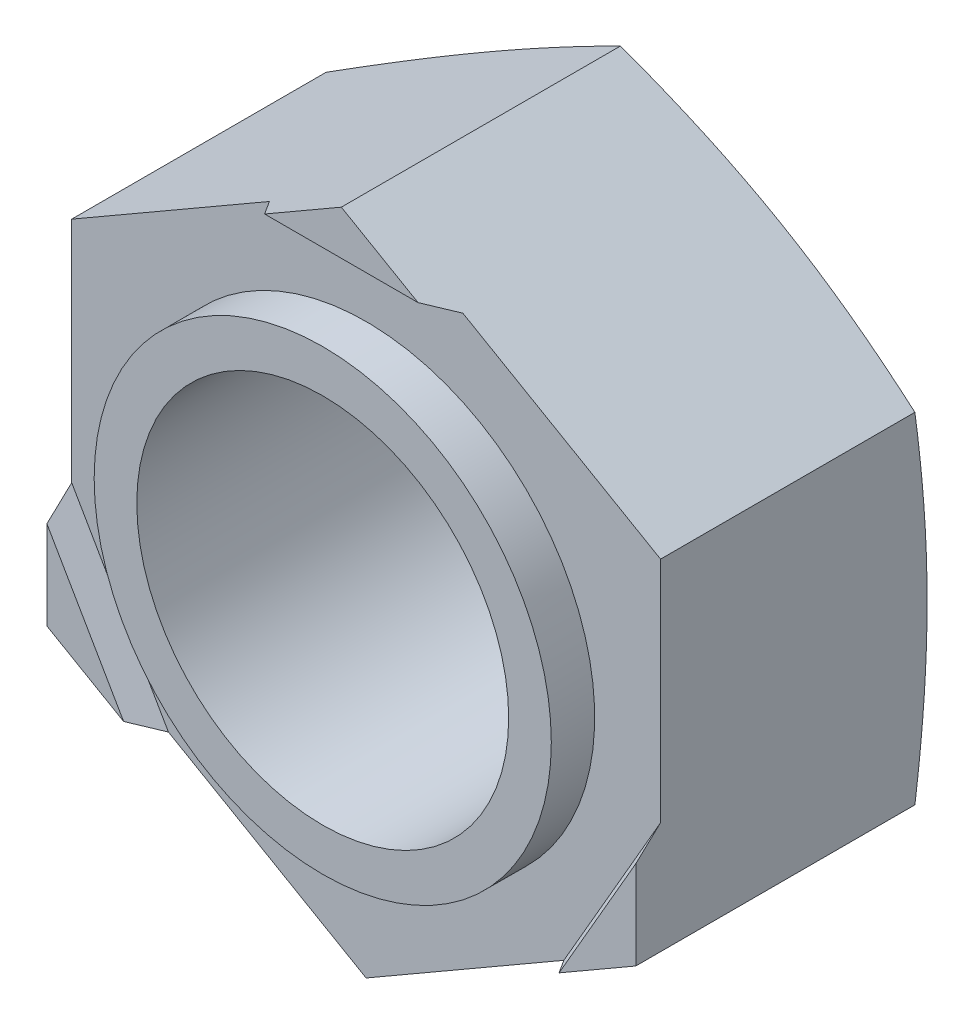
from build123d import *

# Parameters (mm, degrees)
SKETCH_1_R               = 6
EXTRUDE_1_DEPTH          = 10
CUT_EXTRUDE_2_DEPTH      = 18.62337463
PATTERN_CIRCULAR_1_COUNT = 3
SKETCH_2_R               = 7.375
SKETCH_2_R_2             = 6
EXTRUDE_2_DEPTH          = 1.4
SKETCH_4_OUTSIDE_W       = 166.146
SKETCH_4_OUTSIDE_H       = 169.086
SKETCH_4_OUTSIDE_R       = 9.5
CUT_EXTRUDE_3_DEPTH      = 18.62337463
CUT_EXTRUDE_3_DRAFT      = -75
SKETCH_5_R               = 7.535
CUT_EXTRUDE_4_DEPTH      = 0.2


with BuildPart() as part:
    # 草图1 → 拉伸1 (new body)
    with BuildSketch(Plane.XY):
        Polygon((0, 10.969655115), (-9.5, 5.484827557), (-9.5, -5.484827557), (0, -10.969655115), (9.5, -5.484827557), (9.5, 5.484827557), align=None)
        Circle(SKETCH_1_R, mode=Mode.SUBTRACT)
    extrude(amount=EXTRUDE_1_DEPTH)

    # 草图3 → 切除-拉伸2 (cut, symmetric)
    with BuildSketch(Plane(origin=(0, 0, 0), x_dir=(0, 0, -1), z_dir=(1, 0, 0))):
        Polygon((-9.4, 9.540494522), (-8.6, 9.167448395), (-8.6, 0), (-10, 0), (-10, 10.969655115), (-9.4, 10.969655115), align=None)
    cut_extrude_2 = extrude(amount=CUT_EXTRUDE_2_DEPTH, both=True, mode=Mode.SUBTRACT)

    # 阵列(圆周)1: 切除-拉伸2 ×3 about axis
    pattern_circular_1_axis = Axis((0, 0, 0), (0, 0, 1))
    for i in range(1, PATTERN_CIRCULAR_1_COUNT):
        add(cut_extrude_2.rotate(pattern_circular_1_axis, i * 360 / PATTERN_CIRCULAR_1_COUNT), mode=Mode.SUBTRACT)

    # 草图2 → 拉伸2 (add)
    with BuildSketch(Plane.XY.offset(8.6)):
        with Locations(Location((0, 0, 0), (0, 0, 180))):
            Circle(SKETCH_2_R)
        Circle(SKETCH_2_R_2, mode=Mode.SUBTRACT)
    extrude(amount=EXTRUDE_2_DEPTH)


with BuildPart() as cut_extrude_3_tool:
    # 草图4 outside → 切除-拉伸3 (with draft: the straight prism first)
    with BuildSketch(Plane(origin=(0, 0, 0), x_dir=(-1, 0, 0), z_dir=(0, 0, -1))):
        Rectangle(SKETCH_4_OUTSIDE_W, SKETCH_4_OUTSIDE_H)
        Circle(SKETCH_4_OUTSIDE_R, mode=Mode.SUBTRACT)
    extrude(amount=-CUT_EXTRUDE_3_DEPTH)
    # 切除-拉伸3: the draft: its side faces are tilted about the plane it starts from
    cut_extrude_3_sides = [cut_extrude_3_tool.faces().sort_by_distance(p)[0] for p in [
        (0, -84.543, 9.311687315),
        (-83.073, 0, 9.311687315),
        (0, 84.543, 9.311687315),
        (83.073, 0, 9.311687315),
        (9.5, 0, 9.311687315),
    ]]
    draft(cut_extrude_3_sides, Plane(origin=(0, 0, 0), x_dir=(-1, 0, 0), z_dir=(0, 0, -1)), CUT_EXTRUDE_3_DRAFT)


with BuildPart() as part_1:
    add(part.part)

    # 切除-拉伸3: cut by cut_extrude_3_tool
    add(cut_extrude_3_tool.part, mode=Mode.SUBTRACT)

    # 草图5 → 切除-拉伸4 (cut)
    with BuildSketch(Plane(origin=(0, 0, 0), x_dir=(-1, 0, 0), z_dir=(0, 0, -1))):
        Circle(SKETCH_5_R)
    extrude(amount=-CUT_EXTRUDE_4_DEPTH, mode=Mode.SUBTRACT)


solid = part_1.part
